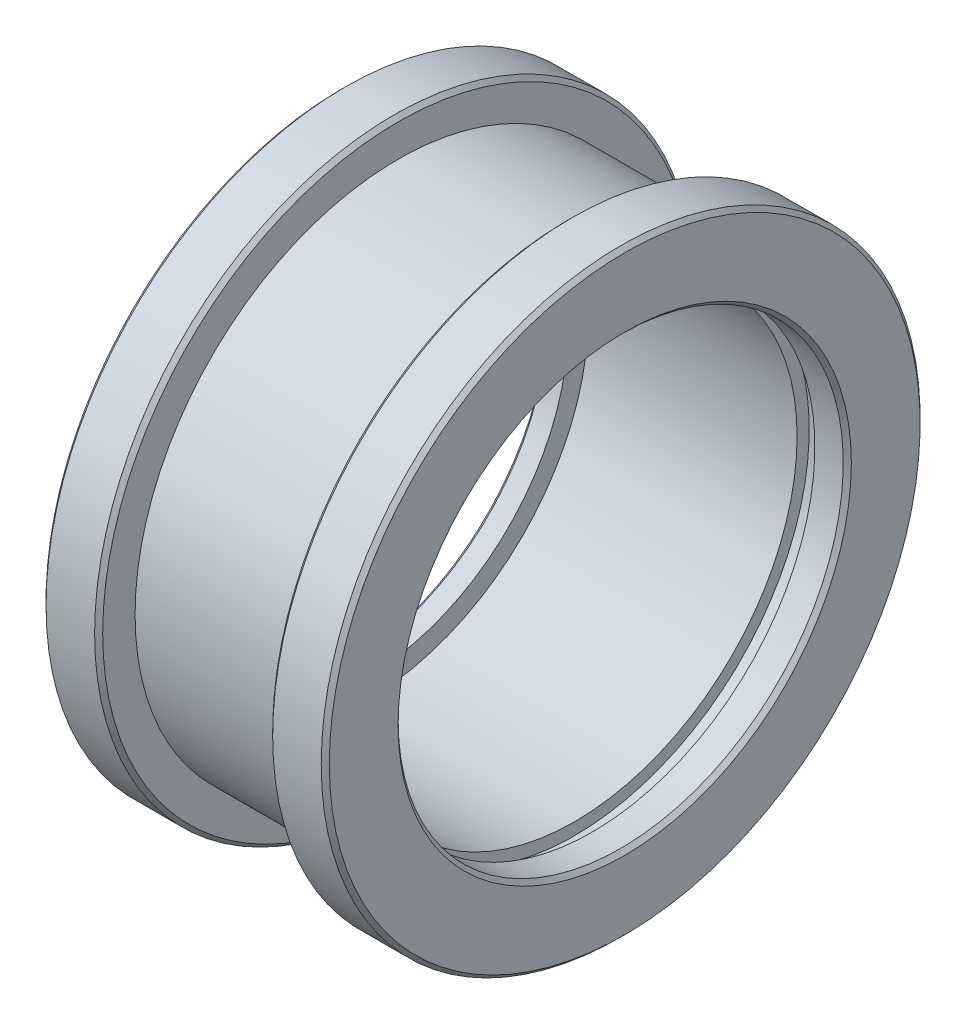
from build123d import *

# Parameters (mm, degrees)
SKETCH_2_R          = 27.5
CUT_EXTRUDE_1_DEPTH = 32
SKETCH_4_R          = 25
CUT_EXTRUDE_2_DEPTH = 30
CHAMFER_1_SIZE      = 0.5
SKETCH_5_W          = 2.2
SKETCH_5_H          = 1.5


with BuildPart() as part:
    # 草图1 → 旋转1 (revolve)
    with BuildSketch(Plane.XY, mode=Mode.PRIVATE) as revolve_1_sk:
        Polygon((-17.5, 0), (17.5, 0), (17.5, 37), (10.5, 37), (10.5, 32.5), (-10.5, 32.5), (-10.5, 37), (-17.5, 37), align=None)
    revolve(revolve_1_sk.sketch.rotate(Axis((-17.5, 0, 0), (1, 0, 0)), 90), axis=Axis((-17.5, 0, 0), (1, 0, 0)))

    # 草图2 → 切除-拉伸1 (cut)
    with BuildSketch(Plane(origin=(17.5, 0, 0), x_dir=(0, 0, -1), z_dir=(1, 0, 0))):
        Circle(SKETCH_2_R)
    extrude(amount=-CUT_EXTRUDE_1_DEPTH, mode=Mode.SUBTRACT)

    # 草图4 → 切除-拉伸2 (cut)
    with BuildSketch(Plane(origin=(-14.5, 0, 0), x_dir=(0, 0, -1), z_dir=(1, 0, 0))):
        Circle(SKETCH_4_R)
    extrude(amount=-CUT_EXTRUDE_2_DEPTH, mode=Mode.SUBTRACT)

    # 倒角1
    chamfer_1_edges = [part.edges().sort_by_distance(p)[0] for p in [
        (17.5, 0, 27.5),
        (-17.5, 0, 25),
        (-17.5, 0, -37),
        (-10.5, 0, -37),
        (10.5, 0, -37),
        (17.5, 0, -37),
    ]]
    chamfer(chamfer_1_edges, length=CHAMFER_1_SIZE)

    # 草图5 → 切除-旋转1 (revolve, cut)
    with BuildSketch(Plane(origin=(0, 0, 0), x_dir=(1, 0, 0), z_dir=(0, 1, 0))):
        with Locations((12.4, 28.25)):
            Rectangle(SKETCH_5_W, SKETCH_5_H)
    revolve(axis=Axis((0, 0, 0), (1, 0, 0)), mode=Mode.SUBTRACT)


solid = part.part
